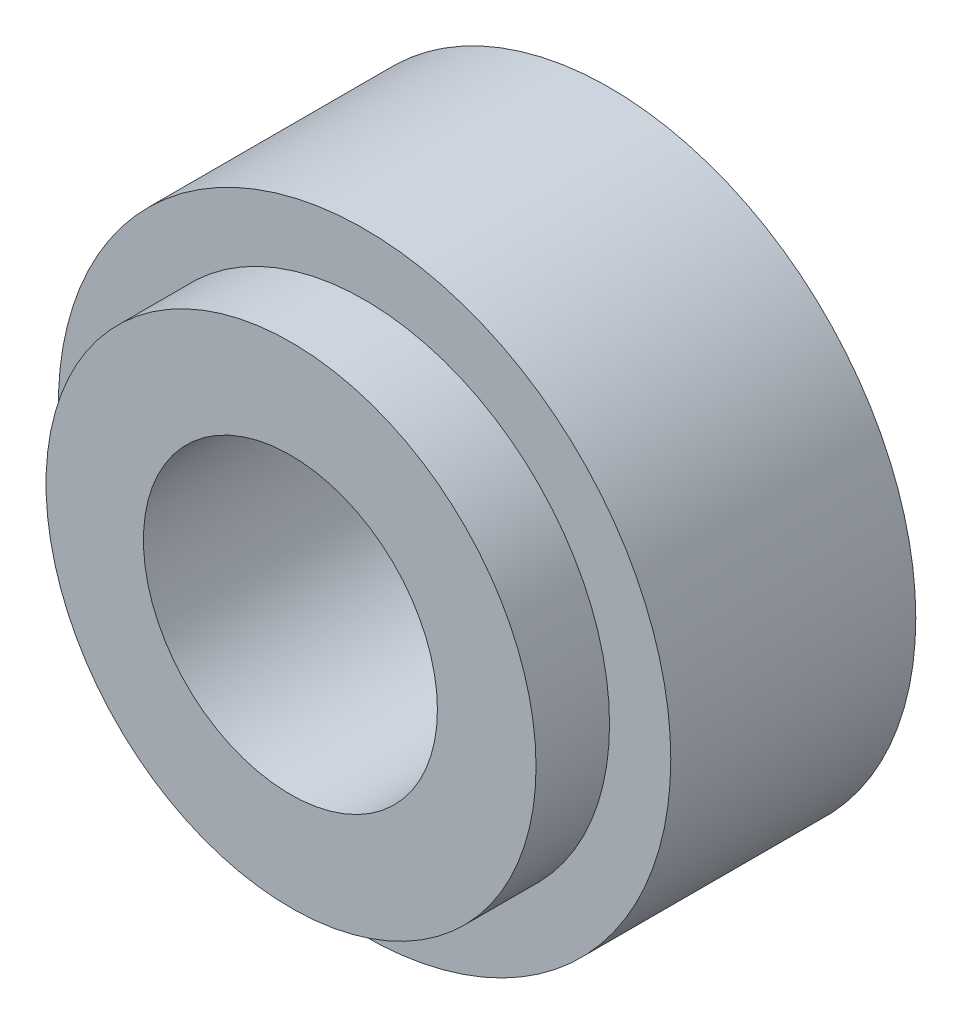
from build123d import *

# Parameters (mm, degrees)
SKETCH1_R              = 12.5
BOSS_EXTRUDE1_DEPTH    = 10
SKETCH2_R              = 10
BOSS_EXTRUDE2_DEPTH    = 3
M14_TAPPED_HOLE1_D     = 12
M14_TAPPED_HOLE1_DEPTH = 34
M14_TAPPED_HOLE1_TIP   = 3.605163714


with BuildPart() as part:
    # Sketch1 → Boss-Extrude1 (new body)
    with BuildSketch(Plane.XY):
        Circle(SKETCH1_R)
    extrude(amount=BOSS_EXTRUDE1_DEPTH)

    # Sketch2 → Boss-Extrude2 (add)
    with BuildSketch(Plane.XY.offset(10)):
        Circle(SKETCH2_R)
    extrude(amount=BOSS_EXTRUDE2_DEPTH)

    # M14 Tapped Hole1
    with Locations(Plane(origin=(-0.024940063, -0.002986858, 13), x_dir=(1, 0, 0), z_dir=(0, 0, 1))):
        with Locations((0, 0)):
            Hole(M14_TAPPED_HOLE1_D / 2, depth=M14_TAPPED_HOLE1_DEPTH)
            with Locations((0, 0, -(M14_TAPPED_HOLE1_DEPTH + M14_TAPPED_HOLE1_TIP / 2))):  # 118° drill point
                Cone(0, M14_TAPPED_HOLE1_D / 2, M14_TAPPED_HOLE1_TIP, mode=Mode.SUBTRACT)


solid = part.part
